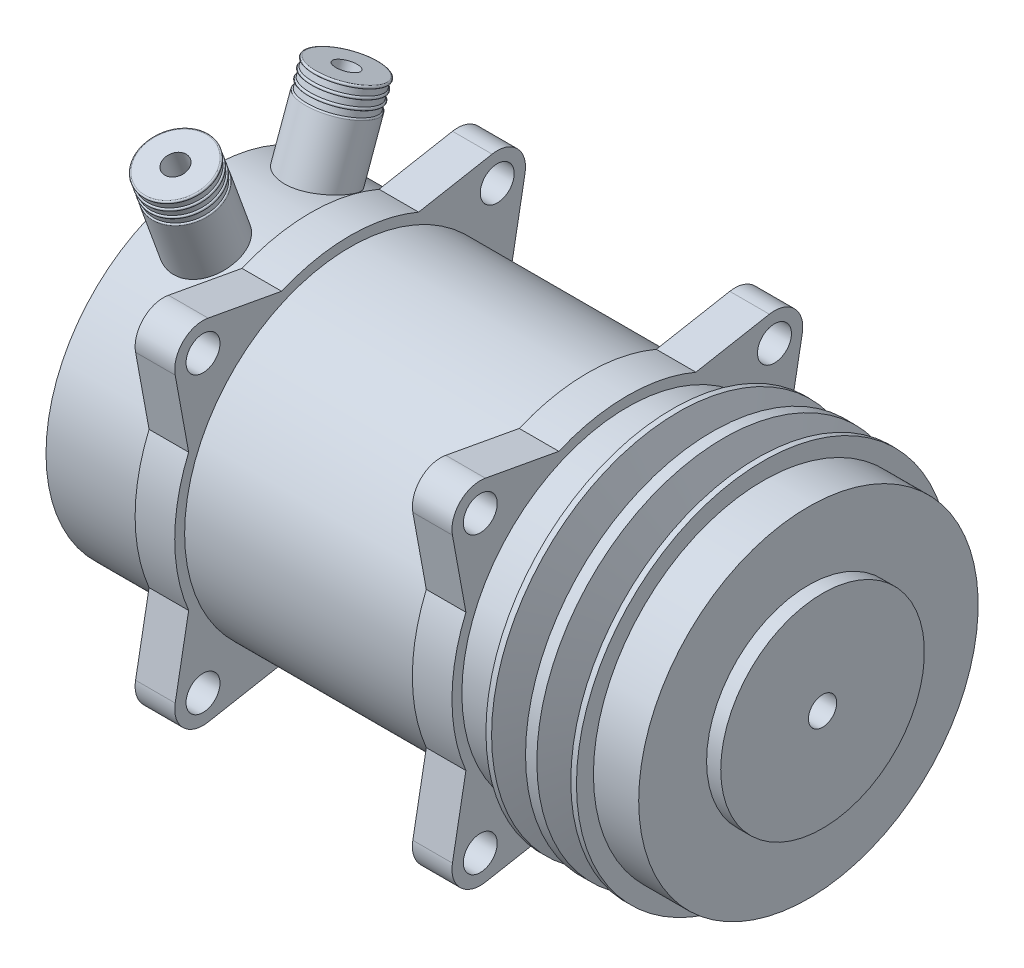
from build123d import *

# Parameters (mm, degrees)
SKETCH1_R                 = 58.5
BOSS_EXTRUDE1_DEPTH       = 147
BOSS_EXTRUDE2_START       = 16
SKETCH2_R                 = 58.5
BOSS_EXTRUDE2_DEPTH       = 16
SKETCH3_W                 = 14
SKETCH3_H                 = 3.5
SKETCH6_R                 = 6
BOSS_EXTRUDE3_DEPTH       = 14
MIRROR3_COPY_1_SKETCH_R   = 6
MIRROR3_COPY_1_DEPTH      = 14
LPATTERN1_COUNT           = 2
LPATTERN1_PITCH           = 98
LPATTERN1_COPY_1_SKETCH_R = 6
LPATTERN1_COPY_1_DEPTH    = 14
LPATTERN1_COPY_2_SKETCH_R = 6
LPATTERN1_COPY_2_DEPTH    = 14
LPATTERN1_COPY_3_SKETCH_R = 6
LPATTERN1_COPY_3_DEPTH    = 14


with BuildPart() as part:
    # Sketch1 → Boss-Extrude1 (new body)
    with BuildSketch(Plane(origin=(0, 0, 0), x_dir=(0, 0, -1), z_dir=(1, 0, 0))):
        Circle(SKETCH1_R)
    extrude(amount=-BOSS_EXTRUDE1_DEPTH)

    # Sketch2 → Boss-Extrude2 (add)
    with BuildSketch(Plane(origin=(0, 0, 0), x_dir=(0, 0, -1), z_dir=(1, 0, 0)).offset(BOSS_EXTRUDE2_START)):
        Circle(SKETCH2_R)
    extrude(amount=-BOSS_EXTRUDE2_DEPTH)

    # Sketch3 → Revolve1 (revolve)
    with BuildSketch(Plane.XY, mode=Mode.PRIVATE) as revolve1_sk:
        Polygon((16, 5), (16, 66), (18, 66), (21.899036355, 54), (26.100963645, 54), (30, 66), (34, 66), (37.899036355, 54), (42.100963645, 54), (46, 66), (48, 66), (48, 60), (64, 60), (64, 36), (69, 36), (69, 5), align=None)
        with Locations((-7, 60.25)):
            Rectangle(SKETCH3_W, SKETCH3_H)
        with Locations((-105, 60.25)):
            Rectangle(SKETCH3_W, SKETCH3_H)
    revolve(revolve1_sk.sketch.rotate(Axis((-162.78049782, 0, 0), (1, 0, 0)), 90), axis=Axis((-162.78049782, 0, 0), (1, 0, 0)))

    # Sketch5 → Revolve2 (revolve)
    with BuildSketch(Plane(origin=(-129.5, 0, 0), x_dir=(0, 0, -1), z_dir=(1, 0, 0))):
        with BuildLine():
            Line((-33.993351153, 81.700747104), (-41.041045809, 79.135596029))
            ThreePointArc((-41.041045809, 79.135596029), (-41.339882048, 78.494739647), (-40.699025666, 78.195903408))
            Line((-40.699025666, 78.195903408), (-40.014985379, 76.316518167))
            ThreePointArc((-40.014985379, 76.316518167), (-40.313821618, 75.675661785), (-39.672965236, 75.376825546))
            Line((-39.672965236, 75.376825546), (-38.988924949, 73.497440305))
            ThreePointArc((-38.988924949, 73.497440305), (-39.287761188, 72.856583922), (-38.646904806, 72.557747684))
            Line((-38.646904806, 72.557747684), (-37.962864519, 70.678362442))
            ThreePointArc((-37.962864519, 70.678362442), (-38.245008341, 70.419825263), (-38.261700758, 70.03750606))
            Line((-38.261700758, 70.03750606), (-27.830086386, 41.376881126))
            Line((-27.830086386, 41.376881126), (-20.31254542, 44.113042273))
            Line((-20.31254542, 44.113042273), (-33.993351153, 81.700747104))
        make_face()
    revolve2 = revolve(axis=Axis((-129.5, 87.36363996, 31.797764503), (0, -0.9396926207859081, -0.34202014332566955)))

    # Mirror1: Revolve2 across plane
    add(revolve2.mirror(Plane.XY))

    # Sketch6 → Boss-Extrude3 (add)
    with BuildSketch(Plane(origin=(0, 0, 0), x_dir=(0, 0, -1), z_dir=(1, 0, 0))):
        with BuildLine():
            Line((-56.389272029, 20.5), (-49.764441168, 13.875169139))
            Line((-49.764441168, 13.875169139), (-13.875169139, 49.764441168))
            Line((-13.875169139, 49.764441168), (-20.5, 56.389272029))
            Line((-20.5, 56.389272029), (-50.195953965, 61.835924863))
            ThreePointArc((-50.195953965, 61.835924863), (-59.071067812, 59.071067812), (-61.835924863, 50.195953965))
            Line((-61.835924863, 50.195953965), (-56.389272029, 20.5))
        make_face()
        with Locations((-52, 52)):
            Circle(SKETCH6_R, mode=Mode.SUBTRACT)
    boss_extrude3 = extrude(amount=-BOSS_EXTRUDE3_DEPTH)

    # Mirror2: Boss-Extrude3 across plane
    add(boss_extrude3.mirror(Plane.XY))

    # Mirror3: Boss-Extrude3 across plane
    add(boss_extrude3.mirror(Plane.ZX))

    # Mirror3 copy 1 sketch → Mirror3 copy 1 (add)
    with BuildSketch(Plane(origin=(0, 0, 0), x_dir=(0, 0, 1), z_dir=(1, 0, 0))):
        with BuildLine():
            Line((-56.389272029, 20.5), (-49.764441168, 13.875169139))
            Line((-49.764441168, 13.875169139), (-13.875169139, 49.764441168))
            Line((-13.875169139, 49.764441168), (-20.5, 56.389272029))
            Line((-20.5, 56.389272029), (-50.195953965, 61.835924863))
            ThreePointArc((-50.195953965, 61.835924863), (-59.071067812, 59.071067812), (-61.835924863, 50.195953965))
            Line((-61.835924863, 50.195953965), (-56.389272029, 20.5))
        make_face()
        with Locations((-52, 52)):
            Circle(MIRROR3_COPY_1_SKETCH_R, mode=Mode.SUBTRACT)
    extrude(amount=-MIRROR3_COPY_1_DEPTH)

    # LPattern1: Boss-Extrude3 ×2
    with Locations(*[(-i * LPATTERN1_PITCH, 0, 0) for i in range(1, LPATTERN1_COUNT)]):
        add(boss_extrude3)

    # LPattern1 copy 1 sketch → LPattern1 copy 1 (add)
    with BuildSketch(Plane(origin=(-98, 0, 0), x_dir=(0, 0, 1), z_dir=(1, 0, 0))):
        with BuildLine():
            Line((-56.389272029, -20.5), (-49.764441168, -13.875169139))
            Line((-49.764441168, -13.875169139), (-13.875169139, -49.764441168))
            Line((-13.875169139, -49.764441168), (-20.5, -56.389272029))
            Line((-20.5, -56.389272029), (-50.195953965, -61.835924863))
            ThreePointArc((-50.195953965, -61.835924863), (-59.071067812, -59.071067812), (-61.835924863, -50.195953965))
            Line((-61.835924863, -50.195953965), (-56.389272029, -20.5))
        make_face()
        with Locations((-52, -52)):
            Circle(LPATTERN1_COPY_1_SKETCH_R, mode=Mode.SUBTRACT)
    extrude(amount=-LPATTERN1_COPY_1_DEPTH)

    # LPattern1 copy 2 sketch → LPattern1 copy 2 (add)
    with BuildSketch(Plane(origin=(-98, 0, 0), x_dir=(0, 0, -1), z_dir=(1, 0, 0))):
        with BuildLine():
            Line((-56.389272029, -20.5), (-49.764441168, -13.875169139))
            Line((-49.764441168, -13.875169139), (-13.875169139, -49.764441168))
            Line((-13.875169139, -49.764441168), (-20.5, -56.389272029))
            Line((-20.5, -56.389272029), (-50.195953965, -61.835924863))
            ThreePointArc((-50.195953965, -61.835924863), (-59.071067812, -59.071067812), (-61.835924863, -50.195953965))
            Line((-61.835924863, -50.195953965), (-56.389272029, -20.5))
        make_face()
        with Locations((-52, -52)):
            Circle(LPATTERN1_COPY_2_SKETCH_R, mode=Mode.SUBTRACT)
    extrude(amount=-LPATTERN1_COPY_2_DEPTH)

    # LPattern1 copy 3 sketch → LPattern1 copy 3 (add)
    with BuildSketch(Plane(origin=(-98, 0, 0), x_dir=(0, 0, 1), z_dir=(1, 0, 0))):
        with BuildLine():
            Line((-56.389272029, 20.5), (-49.764441168, 13.875169139))
            Line((-49.764441168, 13.875169139), (-13.875169139, 49.764441168))
            Line((-13.875169139, 49.764441168), (-20.5, 56.389272029))
            Line((-20.5, 56.389272029), (-50.195953965, 61.835924863))
            ThreePointArc((-50.195953965, 61.835924863), (-59.071067812, 59.071067812), (-61.835924863, 50.195953965))
            Line((-61.835924863, 50.195953965), (-56.389272029, 20.5))
        make_face()
        with Locations((-52, 52)):
            Circle(LPATTERN1_COPY_3_SKETCH_R, mode=Mode.SUBTRACT)
    extrude(amount=-LPATTERN1_COPY_3_DEPTH)


solid = part.part
